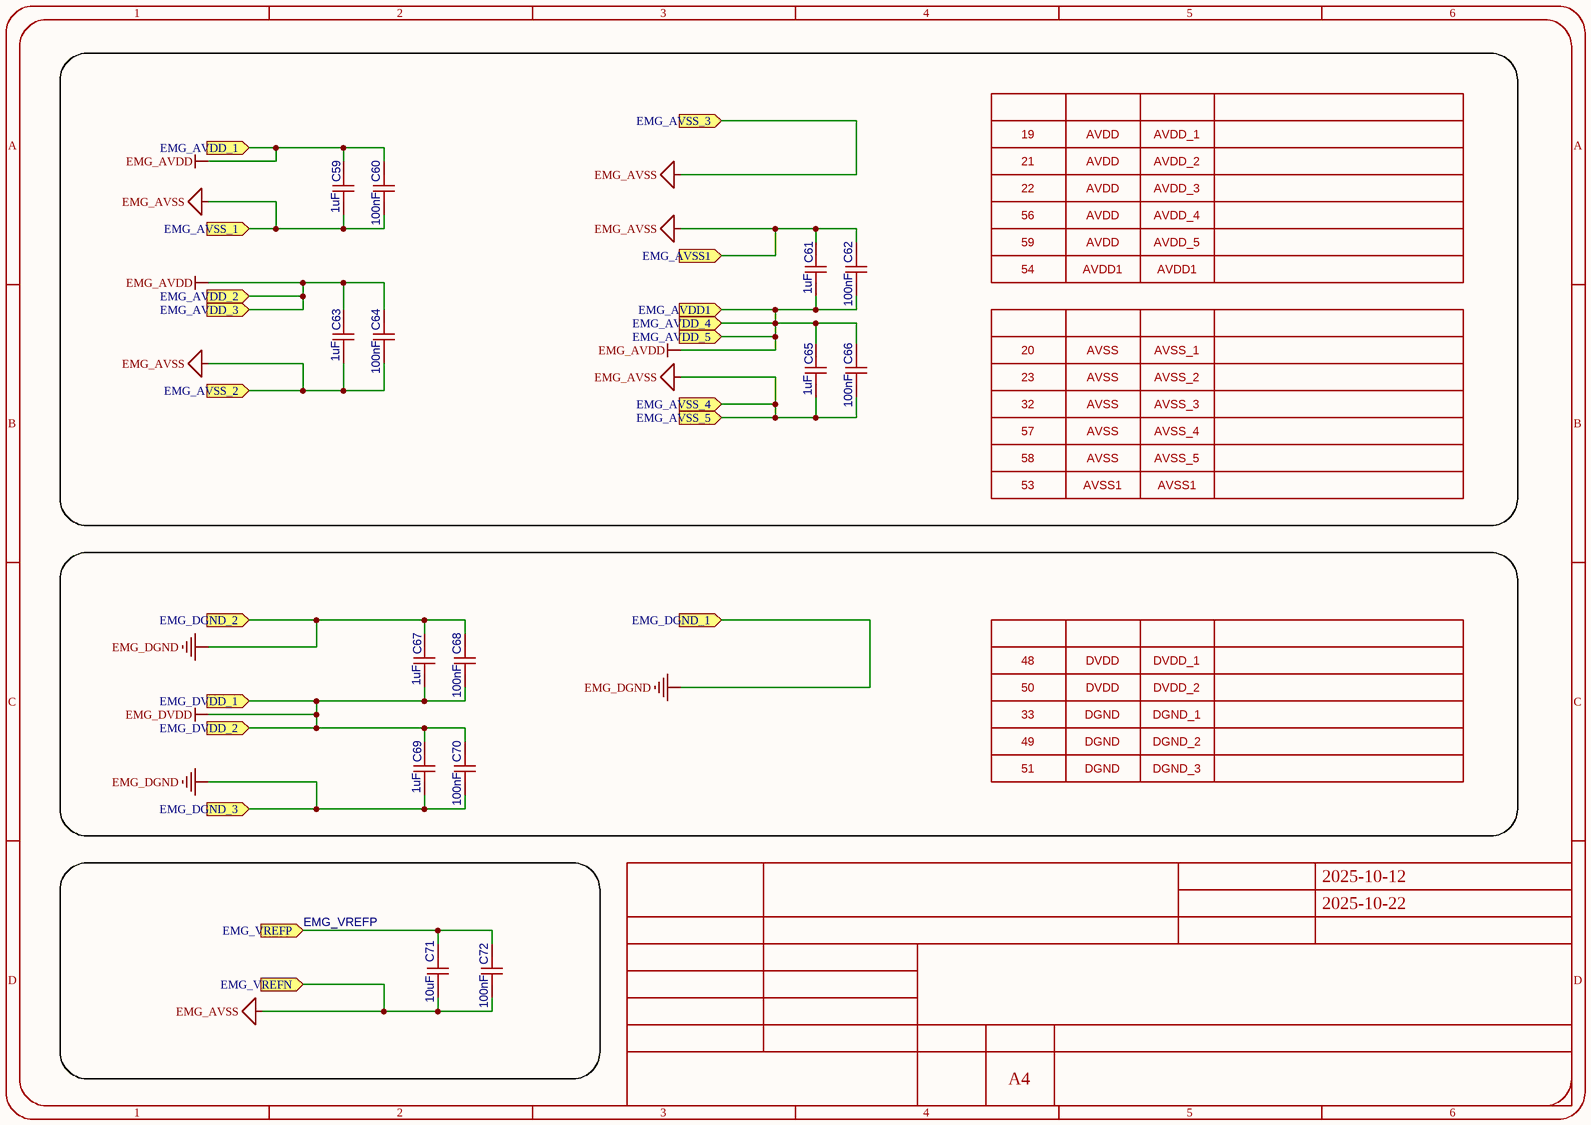
[diagram p0: MISC86293-14.schdoc]
# Altium project MISC86293-17.PrjPCB (part 3 of 3)

## Sheet MISC86293-14.schdoc
size 297 x 209 mm; Version: V1.0; @Project Name: MISC86293; @Page Count: 8; @Update Date: 2025-10-22; @Create Date: 2025-10-12; @Schematic Name: MISC86293; @Page No: 6; @Create Time: 22:53:07; @Update Time: 15:16:24; @Board Name: MISC86293

### Parts
C59  1uF  [C0402]
C60  100nF  [C0402]
C61  1uF  [C0402]
C62  100nF  [C0402]
C63  1uF  [C0402]
C64  100nF  [C0402]
C65  1uF  [C0402]
C66  100nF  [C0402]
C67  1uF  [C0402]
C68  100nF  [C0402]
C69  1uF  [C0402]
C70  100nF  [C0402]
C71  10uF  [C0603]
C72  100nF  [C0402]

### Ports
EMG_AVDD1 (in), EMG_AVDD_1 (in), EMG_AVDD_2 (in), EMG_AVDD_3 (in), EMG_AVDD_4 (in), EMG_AVDD_5 (in), EMG_AVSS1 (in), EMG_AVSS_1 (in), EMG_AVSS_2 (in), EMG_AVSS_3 (in), EMG_AVSS_4 (in), EMG_AVSS_5 (in), EMG_DGND_1 (in), EMG_DGND_2 (in), EMG_DGND_3 (in), EMG_DVDD_1 (in), EMG_DVDD_2 (in), EMG_VREFN (in), EMG_VREFP (in)

### Nets
EMG_AVDD: C59.2 C60.2 C61.1 C62.1 C63.2 C64.2 C65.2 C66.2 ; port EMG_AVDD_1, port EMG_AVDD_2, port EMG_AVDD_3, port EMG_AVDD_4, port EMG_AVDD_5, port EMG_AVDD1  [project net EMG_AVDD1]
EMG_AVSS: C59.1 C60.1 C61.2 C62.2 C63.1 C64.1 C65.1 C66.1 C71.1 C72.1 ; port EMG_AVSS_1, port EMG_AVSS_2, port EMG_AVSS_3, port EMG_AVSS_4, port EMG_AVSS_5, port EMG_VREFN, port EMG_AVSS1  [project net EMG_AVSS1]
EMG_DGND: C67.2 C68.2 C69.1 C70.1 ; port EMG_DGND_1, port EMG_DGND_2, port EMG_DGND_3  [project net EMG_DGND_1]
EMG_DVDD: C67.1 C68.1 C69.2 C70.2 ; port EMG_DVDD_2, port EMG_DVDD_1  [project net EMG_DVDD_1]
EMG_VREFP: C71.2 C72.2 ; port EMG_VREFP

### Notes on the sheet
- 19
- AVDD
- AVDD_1
- 21
- 22
- AVDD_2
- AVDD_3
- 56
- 59
- 54
- AVDD1
- AVDD_4
- AVDD_5
- 20
- 23
- 32
- AVSS
- AVSS_1
- AVSS_2
- AVSS_3
- 57
- 58
- AVSS_4
- AVSS_5
- 53
- AVSS1
- 48
- DVDD
- DVDD_1
- 50
- 33
- 49
- DGND
- DVDD_2
- DGND_1
- DGND_2
- 51
- DGND_3
- 1
- 2
- 3
- 4
- 5
- 6
- A
- B
- C
- 2025-10-12
- 2025-10-22
- D
- A4

### Library data of the parts
C59 C61 C63 C65 C67 C69 = GRM155Z71A105KE01D: AddInBom: yes; ModelId: 36a51122f27c49738f86b3bfa98863e0; ModelName: C0402_L1.0-W0.5-H0.5; ModelTransform: 39.37,19.685,0,0,0,0,0,0,0; Voltage Rated: 10V; Temperature Coefficient: X7R; Symbol: GRM155Z71A105KE01D; Device: GRM155Z71A105KE01D; SupplierPart: C528974; ManufacturerPart: GRM155Z71A105KE01D; Supplier Footprint: 0402; Datasheet: https://atta.szlcsc.com/upload/public/pdf/source/20200508/C528974_15BC5D9F0CC13FAE313D74FE55DE6D9B.pdf; Supplier: LCSC; ConvertToPcb: yes; FootprintName: C0402; Value: 1uF
C60 C62 C64 C66 C68 C70 C72 = CL05B104KB54PNC: AddInBom: yes; ModelId: 36a51122f27c49738f86b3bfa98863e0; ModelName: C0402_L1.0-W0.5-H0.5; ModelTransform: 39.37,19.685,0,0,0,0,0,0,0; Voltage Rated: 50V; Temperature Coefficient: X7R; Device: CL05B104KB54PNC; Symbol: CL05B104KB54PNC; SupplierPart: C307331; ManufacturerPart: CL05B104KB54PNC; Supplier Footprint: 0402; Datasheet: https://atta.szlcsc.com/upload/public/pdf/source/20160218/1457707763339.pdf; Supplier: LCSC; ConvertToPcb: yes; FootprintName: C0402; Value: 100nF
C71 = CL10A106MA8NRNC: AddInBom: yes; ModelId: ac125912035d415993ca9572d50418b1; ModelName: C0603_L1.6-W0.8-H0.8; ModelTransform: 62.992,31.496,0,0,0,0,0,0,0; Voltage Rated: 25V; Temperature Coefficient: X5R; Symbol: CL10A106MA8NRNC; Device: CL10A106MA8NRNC; Supplier: LCSC; Manufacturer Part: CL10A106MA8NRNC; Value: 10uF; Supplier Part: C96446; Supplier Footprint: 0603; Datasheet: https://atta.szlcsc.com/upload/public/pdf/source/20160218/1457707763339.pdf; ConvertToPcb: yes; FootprintName: C0603

## Sheet MISC86293-10.schdoc
size 297 x 209 mm; Version: V1.0; @Project Name: MISC86293; @Page Count: 8; @Update Date: 2025-10-25; @Create Date: 2025-10-24; @Schematic Name: MISC86293; @Page No: 5; @Create Time: 20:02:05; @Update Time: 11:40:48; @Board Name: MISC86293
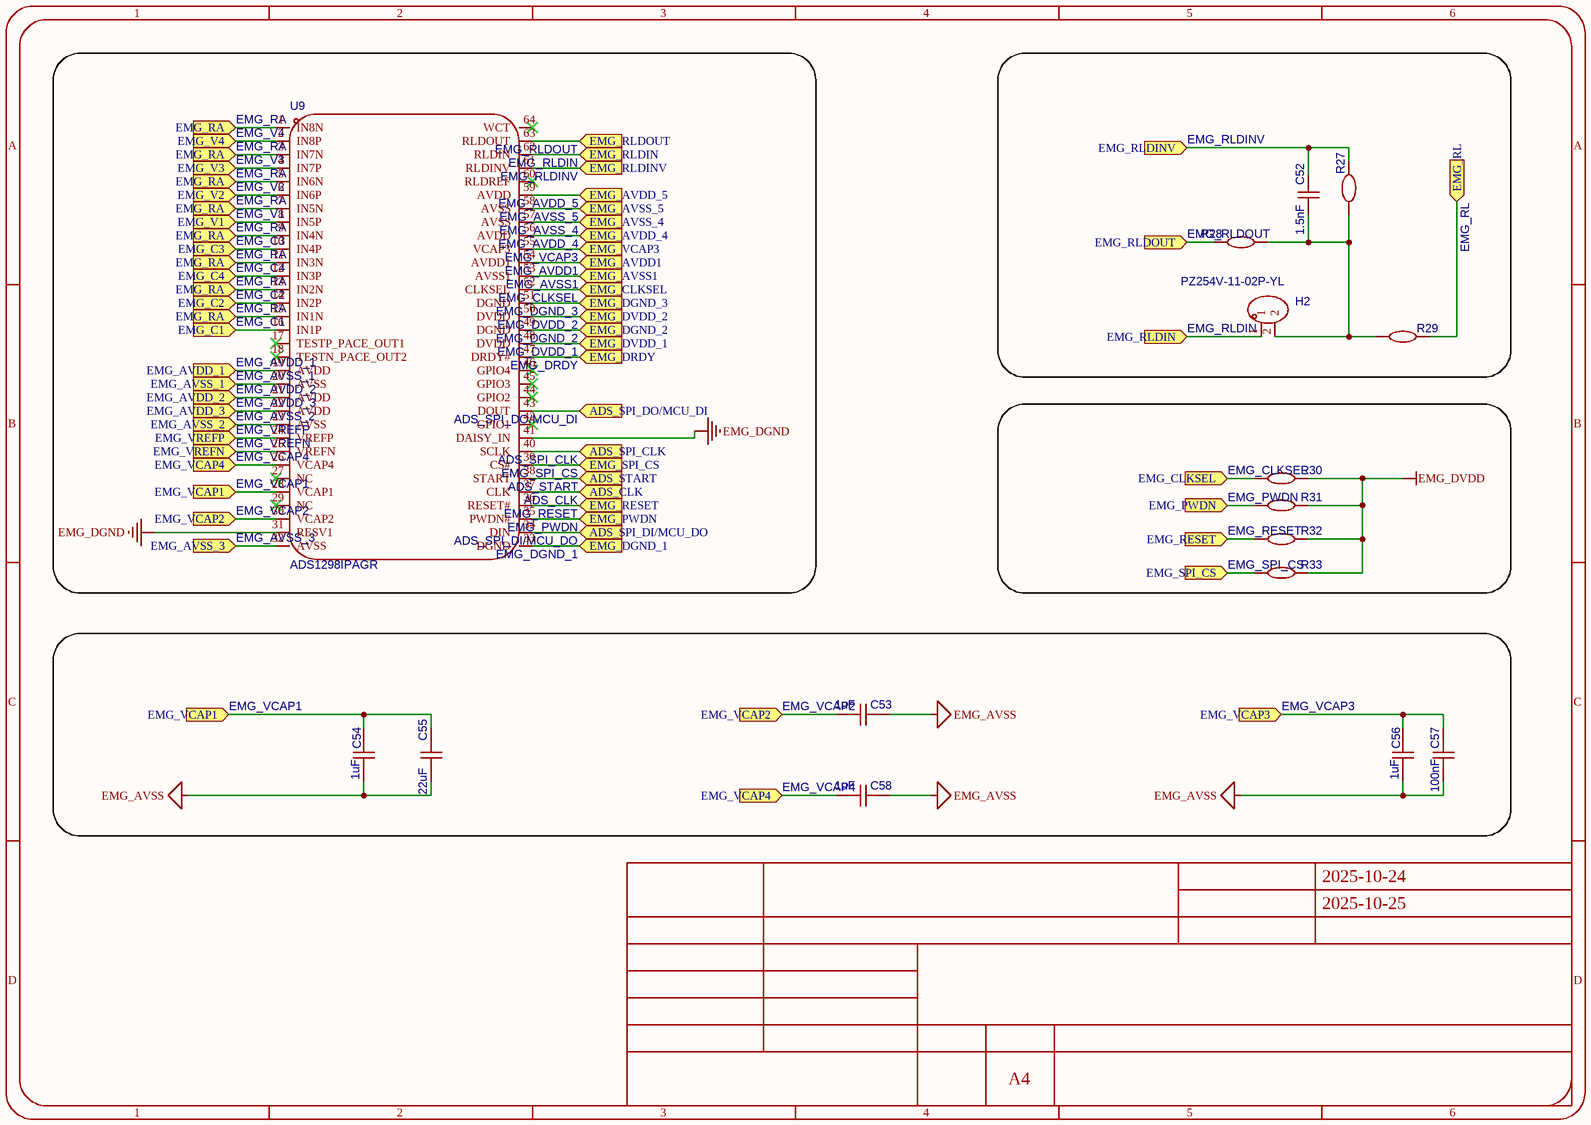
[diagram p1: MISC86293-10.schdoc]

### Parts
C52  1.5nF  [C0402]
C53  1uF  [C0402]
C54  1uF  [C0402]
C55  22uF  [C1206]
C56  1uF  [C0402]
C57  100nF  [C0402]
C58  1uF  [C0402]
H2  PZ254V-11-02P-YL  [HDR-TH_2P-P2.54-V-M]
R27  (no value)  [R0402]
R28  (no value)  [R0402]
R29  (no value)  [R0402]
R30  (no value)  [R0402]
R31  (no value)  [R0402]
R32  (no value)  [R0402]
R33  (no value)  [R0402]
U9  ADS1298IPAGR  [TQFP-64_L10.0-W10.0-P0.50-LS12.0-BL]

### Ports
ADS_CLK (in), ADS_SPI_CLK (in), ADS_SPI_DI/MCU_DO (in), ADS_SPI_DO/MCU_DI (in), ADS_START (in), EMG_AVDD1 (in), EMG_AVDD_1 (in), EMG_AVDD_2 (in), EMG_AVDD_3 (in), EMG_AVDD_4 (in), EMG_AVDD_5 (in), EMG_AVSS1 (in), EMG_AVSS_1 (in), EMG_AVSS_2 (in), EMG_AVSS_3 (in), EMG_AVSS_4 (in), EMG_AVSS_5 (in), EMG_C1 (in), EMG_C2 (in), EMG_C3 (in), EMG_C4 (in), EMG_CLKSEL (in), EMG_DGND_1 (in), EMG_DGND_2 (in), EMG_DGND_3 (in), EMG_DRDY (in), EMG_DVDD_1 (in), EMG_DVDD_2 (in), EMG_PWDN (in), EMG_RA (in), EMG_RESET (in), EMG_RL (in), EMG_RLDIN (in), EMG_RLDINV (in), EMG_RLDOUT (in), EMG_SPI_CS (in), EMG_V1 (in), EMG_V2 (in), EMG_V3 (in), EMG_V4 (in), EMG_VCAP1 (in), EMG_VCAP2 (in), EMG_VCAP3 (in), EMG_VCAP4 (in), EMG_VREFN (in), EMG_VREFP (in)

### Nets
EMG_AVDD1: U9.19(AVDD) U9.21(AVDD) U9.22(AVDD) U9.54(AVDD1) U9.56(AVDD) U9.59(AVDD) ; port EMG_AVDD_5, port EMG_AVDD1, port EMG_AVDD_4, port EMG_AVDD_1, port EMG_AVDD_2, port EMG_AVDD_3  [also labelled EMG_AVDD_1, EMG_AVDD_2, EMG_AVDD_3, EMG_AVDD_4, EMG_AVDD_5]
EMG_AVSS1: C53.2 C54.1 C55.1 C56.1 C57.1 C58.2 U9.20(AVSS) U9.23(AVSS) U9.25(VREFN) U9.32(AVSS) U9.53(AVSS1) U9.57(AVSS) U9.58(AVSS) ; port EMG_AVSS_5, port EMG_AVSS_4, port EMG_AVSS1, port EMG_AVSS_1, port EMG_AVSS_2, port EMG_VREFN, port EMG_AVSS_3  [also labelled EMG_AVSS, EMG_AVSS_1, EMG_AVSS_2, EMG_AVSS_3, EMG_AVSS_4, EMG_AVSS_5, EMG_VREFN]
EMG_DGND_1: U9.31(RESV1) U9.33(DGND) U9.41(DAISY_IN) U9.49(DGND) U9.51(DGND) ; port EMG_DGND_2, port EMG_DGND_3, port EMG_DGND_1  [also labelled EMG_DGND, EMG_DGND_2, EMG_DGND_3]
EMG_DVDD_1: R30.2 R31.2 R32.2 R33.2 U9.48(DVDD) U9.50(DVDD) ; port EMG_DVDD_2, port EMG_DVDD_1  [also labelled EMG_DVDD, EMG_DVDD_2]
ADS_CLK: U9.37(CLK) ; port ADS_CLK
ADS_SPI_CLK: U9.40(SCLK) ; port ADS_SPI_CLK
ADS_SPI_DI/MCU_DO: U9.34(DIN) ; port ADS_SPI_DI/MCU_DO
ADS_SPI_DO/MCU_DI: U9.43(DOUT) ; port ADS_SPI_DO/MCU_DI
ADS_START: U9.38(START) ; port ADS_START
EMG_C1: U9.16(IN1P) ; port EMG_C1
EMG_C2: U9.14(IN2P) ; port EMG_C2
EMG_C3: U9.10(IN4P) ; port EMG_C3
EMG_C4: U9.12(IN3P) ; port EMG_C4
EMG_CLKSEL: R30.1 U9.52(CLKSEL) ; port EMG_CLKSEL
EMG_DRDY: U9.47(DRDY#) ; port EMG_DRDY
EMG_PWDN: R31.1 U9.35(PWDN#) ; port EMG_PWDN
EMG_RA: U9.1(IN8N) U9.3(IN7N) U9.5(IN6N) U9.7(IN5N) U9.9(IN4N) U9.11(IN3N) U9.13(IN2N) U9.15(IN1N) ; port EMG_RA
EMG_RESET: R32.1 U9.36(RESET#) ; port EMG_RESET
EMG_RL: R29.2 ; port EMG_RL
EMG_RLDIN: H2.1 U9.62(RLDIN) ; port EMG_RLDIN
EMG_RLDINV: C52.2 R27.1 U9.61(RLDINV) ; port EMG_RLDINV
EMG_RLDOUT: R28.1 U9.63(RLDOUT) ; port EMG_RLDOUT
EMG_SPI_CS: R33.1 U9.39(CS#) ; port EMG_SPI_CS
EMG_V1: U9.8(IN5P) ; port EMG_V1
EMG_V2: U9.6(IN6P) ; port EMG_V2
EMG_V3: U9.4(IN7P) ; port EMG_V3
EMG_V4: U9.2(IN8P) ; port EMG_V4
EMG_VCAP1: C54.2 C55.2 U9.28(VCAP1) ; port EMG_VCAP1
EMG_VCAP2: C53.1 U9.30(VCAP2) ; port EMG_VCAP2
EMG_VCAP3: C56.2 C57.2 U9.55(VCAP3) ; port EMG_VCAP3
EMG_VCAP4: C58.1 U9.26(VCAP4) ; port EMG_VCAP4
EMG_VREFP: U9.24(VREFP) ; port EMG_VREFP
NetC52_1: C52.1 H2.2 R27.2 R28.2 R29.1

Not connected (* = marked no-connect by the designer): U9 17(TESTP_PACE_OUT1)* 18(TESTN_PACE_OUT2)* 27(NC)* 29(NC)* 42(GPIO1)* 44(GPIO2)* 45(GPIO3)* 46(GPIO4)* 60(RLDREF)* 64(WCT)*

### Notes on the sheet
- 1
- 2
- 3
- 4
- 5
- 6
- A
- B
- C
- 2025-10-24
- 2025-10-25
- D
- A4

### Library data of the parts
C52 = CC0402KRX7R9BB152: AddInBom: yes; ModelId: 36a51122f27c49738f86b3bfa98863e0; ModelName: C0402_L1.0-W0.5-H0.5; ModelTransform: 39.37,19.685,0,0,0,0,0,0,0; Voltage Rated: 50V; Temperature Coefficient: X7R; Symbol: CC0402KRX7R9BB152; Device: CC0402KRX7R9BB152; Supplier: LCSC; Manufacturer Part: CC0402KRX7R9BB152; Value: 1.5nF; Supplier Part: C107022; Supplier Footprint: 0402; Datasheet: https://atta.szlcsc.com/upload/public/pdf/source/20170914/C128857_1505359892143968080.pdf; ConvertToPcb: yes; FootprintName: C0402
C53 C54 C56 C58 = GRM155Z71A105KE01D: as C59 on sheet MISC86293-14; Symbol: GRM155Z71A105KE01D; Device: GRM155Z71A105KE01D; SupplierPart: C528974; ManufacturerPart: GRM155Z71A105KE01D; Supplier Footprint: 0402; Datasheet: https://atta.szlcsc.com/upload/public/pdf/source/20200508/C528974_15BC5D9F0CC13FAE313D74FE55DE6D9B.pdf; Supplier: LCSC; ConvertToPcb: yes; FootprintName: C0402; Value: 1uF
C55 = CL31A226KAHNNNE: Symbol: GRM31CR61A107ME05L; AddInBom: yes; ModelId: e4be705b945545a48e666415e3682bd8; ModelName: C1206_L3.2-W1.6-H1.3; ModelTransform: 125.984,62.992,0,0,0,0,0,0,0; Voltage Rating: 25V; Temperature Coefficient: X5R; Device: CL31A226KAHNNNE; Supplier: LCSC; Supplier Part: C12891; Manufacturer Part: CL31A226KAHNNNE; Value: 22uF; JLCPCB Part Class: Basic Part; Supplier Footprint: 1206; Datasheet: https://item.szlcsc.com/datasheet/CL31A226KAHNNNE/13537.html; ConvertToPcb: yes; FootprintName: C1206
C57 = CL05B104KB54PNC: as C60 on sheet MISC86293-14; Device: CL05B104KB54PNC; Symbol: CL05B104KB54PNC; SupplierPart: C307331; ManufacturerPart: CL05B104KB54PNC; Supplier Footprint: 0402; Datasheet: https://atta.szlcsc.com/upload/public/pdf/source/20160218/1457707763339.pdf; Supplier: LCSC; ConvertToPcb: yes; FootprintName: C0402; Value: 100nF
H2 = PZ254V-11-02P-YL: AddInBom: yes; ModelId: e35305ec3aa84b66b849f914b715e73f; ModelName: HDR2.54-M-LI-1X2P; ModelTransform: 200,100,0,0,0,0,0,0,-118.11; Pin Structure: 1x2P; Pitch: 2.54mm; Current Rating: 3A; Symbol: PZ254V-11-02P-YL; Device: PZ254V-11-02P-YL; SupplierPart: C41425305; ManufacturerPart: PZ254V-11-02P-YL; Datasheet: https://item.szlcsc.com/datasheet/PZ254V-11-02P-YL/43268222.html; Supplier: LCSC; ConvertToPcb: yes; FootprintName: HDR-TH_2P-P2.54-V-M; Number of Pins: 2P; Length of Mating Pin: 6.1mm; Insulation Height: 2.5mm; Length of End Connection Pin: 3mm
R27 = SC0402F1004F2ANRH: AddInBom: yes; ModelId: 671aefced39d4c318694bba8bd8efd39; ModelName: R0402_L1.0-W0.5-H0.5; ModelTransform: 39.37,19.685,0,0,0,0,0,0.0005,0; Symbol: SC0402F1004F2ANRH; Device: SC0402F1004F2ANRH; SupplierPart: C3152068; ManufacturerPart: SC0402F1004F2ANRH; Supplier Footprint: 0402; Datasheet: https://atta.szlcsc.com/upload/public/pdf/source/20220728/FFCE43BB6DF8FA16AEE331F0F4B289DE.pdf; Supplier: LCSC; ConvertToPcb: yes; FootprintName: R0402; Power(Watts): -
R28 = 0402WGF0000TCE: AddInBom: yes; ModelId: 671aefced39d4c318694bba8bd8efd39; ModelName: R0402_L1.0-W0.5-H0.5; ModelTransform: 39.37,19.685,0,0,0,0,0,0.0005,0; Power(Watts): 62.5mW; Overload Voltage (Max): 50V; Symbol: 0402WGF0000TCE; Device: 0402WGF0000TCE; Supplier: LCSC; Manufacturer Part: 0402WGF0000TCE; Supplier Part: C17168; Supplier Footprint: 0402; Datasheet: https://atta.szlcsc.com/upload/public/pdf/source/20200306/C422600_1E6D84923E4A46A82E41ADD87F860B5C.pdf; ConvertToPcb: yes; FootprintName: R0402
R29 = RC0402FR-07100KL: AddInBom: yes; ModelId: 671aefced39d4c318694bba8bd8efd39; ModelName: R0402_L1.0-W0.5-H0.5; ModelTransform: 39.37,19.685,0,0,0,0,0,0.0005,0; Power(Watts): 62.5mW; Overload Voltage (Max): 50V; Device: RC0402FR-07100KL; Symbol: RC0402FR-07100KL; SupplierPart: C60491; ManufacturerPart: RC0402FR-07100KL; Supplier Footprint: 0402; JLCPCB Part Class: Extended Part; Datasheet: https://atta.szlcsc.com/upload/public/pdf/source/20180927/C295883_E8D83085EA81BD7DE0B2B681138C15EE.pdf; Supplier: LCSC; ConvertToPcb: yes; FootprintName: R0402
R30-R33 = RC0402FR-0710KL: AddInBom: yes; ModelId: 671aefced39d4c318694bba8bd8efd39; ModelName: R0402_L1.0-W0.5-H0.5; ModelTransform: 39.37,19.685,0,0,0,0,0,0.0005,0; Power(Watts): 62.5mW; Overload Voltage (Max): 50V; Symbol: RC0402FR-0710KL; Device: RC0402FR-0710KL; SupplierPart: C60490; ManufacturerPart: RC0402FR-0710KL; Supplier Footprint: 0402; Datasheet: https://atta.szlcsc.com/upload/public/pdf/source/20170925/C131467_1506321478108990263.pdf; Supplier: LCSC; ConvertToPcb: yes; FootprintName: R0402
U9 = ADS1298IPAGR: AddInBom: yes; ModelId: 8d2ba6bfb2a14fb7921a74871619a185; ModelName: TQFP-64_L10.0-W10.0-H1.2-LS12.0-P0.50; ModelTransform: 473.00941,473.00941,0,90,0,0,0,0.039,0; Symbol: ADS1298IPAGR; Device: ADS1298IPAGR; SupplierPart: C527440; ManufacturerPart: ADS1298IPAGR; Supplier Footprint: TQFP-64(10x10); Datasheet: https://www.ti.com/cn/lit/gpn/ads1298; Supplier: LCSC; ConvertToPcb: yes; FootprintName: TQFP-64_L10.0-W10.0-P0.50-LS12.0-BL

## Nets that join several sheets
EEG_AVDD1: MISC86293-47 (L3.2), MISC86293-8 (8 pins), MISC86293-4 (7 pins)
EEG_AVSS1: MISC86293-47 (R6.1), MISC86293-6 (16 pins), MISC86293-8 (10 pins), MISC86293-4 (13 pins)
EEG_DGND_1: MISC86293-47 (R58.1), MISC86293-8 (C38.2 C39.2 C40.1 C41.1), MISC86293-4 (9 pins)
EEG_DVDD_1: MISC86293-47 (L4.2), MISC86293-8 (C38.1 C39.1 C40.2 C41.2), MISC86293-4 (6 pins)
EMG_AVDD1: MISC86293-47 (L2.2), MISC86293-14 (8 pins), MISC86293-10 (6 pins)
EMG_AVSS1: MISC86293-47 (R7.1), MISC86293-12 (30 pins), MISC86293-14 (10 pins), MISC86293-10 (13 pins)
EMG_DGND_1: MISC86293-47 (R59.1), MISC86293-14 (C67.2 C68.2 C69.1 C70.1), MISC86293-10 (5 pins)
EMG_DVDD_1: MISC86293-47 (L5.2), MISC86293-14 (C67.1 C68.1 C69.2 C70.2), MISC86293-10 (6 pins)
SIGNAL_GND: MISC86293-47 (34 pins), MISC86293-21 (24 pins)
STM_VCC3V3: MISC86293-47 (L6.2), MISC86293-21 (19 pins)
ADS_CLK: MISC86293-4 (U8.37), MISC86293-10 (U9.37)
ADS_SPI_CLK: MISC86293-4 (U8.40), MISC86293-21 (U10.30), MISC86293-10 (U9.40)
ADS_SPI_DI/MCU_DO: MISC86293-4 (U8.34), MISC86293-21 (U10.32), MISC86293-10 (U9.34)
ADS_SPI_DO/MCU_DI: MISC86293-4 (U8.43), MISC86293-21 (U10.31), MISC86293-10 (U9.43)
ADS_START: MISC86293-4 (U8.38), MISC86293-21 (U10.26), MISC86293-10 (U9.38)
EEG_A1: MISC86293-6 (C50.2 R25.2), MISC86293-4 (U8.8)
EEG_BIAS: MISC86293-6 (C44.2 R19.2), MISC86293-4 (R10.2)
EEG_CLKSEL: MISC86293-4 (R15.1 U8.52), MISC86293-21 (U10.98)
EEG_CZ: MISC86293-6 (C49.2 R24.2), MISC86293-4 (U8.10)
EEG_DRDY: MISC86293-4 (U8.47), MISC86293-21 (U10.1)
EEG_EOGN: MISC86293-6 (C47.2 R22.2), MISC86293-4 (U8.16)
EEG_EOGP: MISC86293-6 (C46.2 R21.2), MISC86293-4 (U8.14)
EEG_FZ: MISC86293-6 (C48.2 R23.2), MISC86293-4 (U8.12)
EEG_PWDN: MISC86293-4 (R16.1 U8.35), MISC86293-21 (U10.4)
EEG_PZ: MISC86293-6 (C51.2 R26.2), MISC86293-4 (U8.6)
EEG_REF: MISC86293-6 (C45.2 R20.2), MISC86293-4 (U8.17)
EEG_RESET: MISC86293-4 (R17.1 U8.36), MISC86293-21 (U10.3)
EEG_SPI_CS: MISC86293-4 (R18.1 U8.39), MISC86293-21 (U10.2)
EEG_VREFP: MISC86293-8 (C42.2 C43.2), MISC86293-4 (U8.24)
EMG_C1: MISC86293-12 (C74.2 R35.2), MISC86293-10 (U9.16)
EMG_C2: MISC86293-12 (C76.2 R37.2), MISC86293-10 (U9.14)
EMG_C3: MISC86293-12 (C78.2 R39.2), MISC86293-10 (U9.10)
EMG_C4: MISC86293-12 (C80.2 R41.2), MISC86293-10 (U9.12)
EMG_CLKSEL: MISC86293-21 (U10.38), MISC86293-10 (R30.1 U9.52)
EMG_DRDY: MISC86293-21 (U10.39), MISC86293-10 (U9.47)
EMG_PWDN: MISC86293-21 (U10.42), MISC86293-10 (R31.1 U9.35)
EMG_RA: MISC86293-12 (C90.2 R51.2), MISC86293-10 (8 pins)
EMG_RESET: MISC86293-21 (U10.41), MISC86293-10 (R32.1 U9.36)
EMG_RL: MISC86293-12 (C92.2 R53.2), MISC86293-10 (R29.2)
EMG_SPI_CS: MISC86293-21 (U10.40), MISC86293-10 (R33.1 U9.39)
EMG_V1: MISC86293-12 (C82.2 R43.2), MISC86293-10 (U9.8)
EMG_V2: MISC86293-12 (C84.2 R45.2), MISC86293-10 (U9.6)
EMG_V3: MISC86293-12 (C86.2 R47.2), MISC86293-10 (U9.4)
EMG_V4: MISC86293-12 (C88.2 R49.2), MISC86293-10 (U9.2)
EMG_VREFP: MISC86293-14 (C71.2 C72.2), MISC86293-10 (U9.24)
RAW_STM32_RX: MISC86293-47 (U5.6), MISC86293-21 (U10.87)
RAW_STM32_TX: MISC86293-47 (U5.7), MISC86293-21 (U10.86)